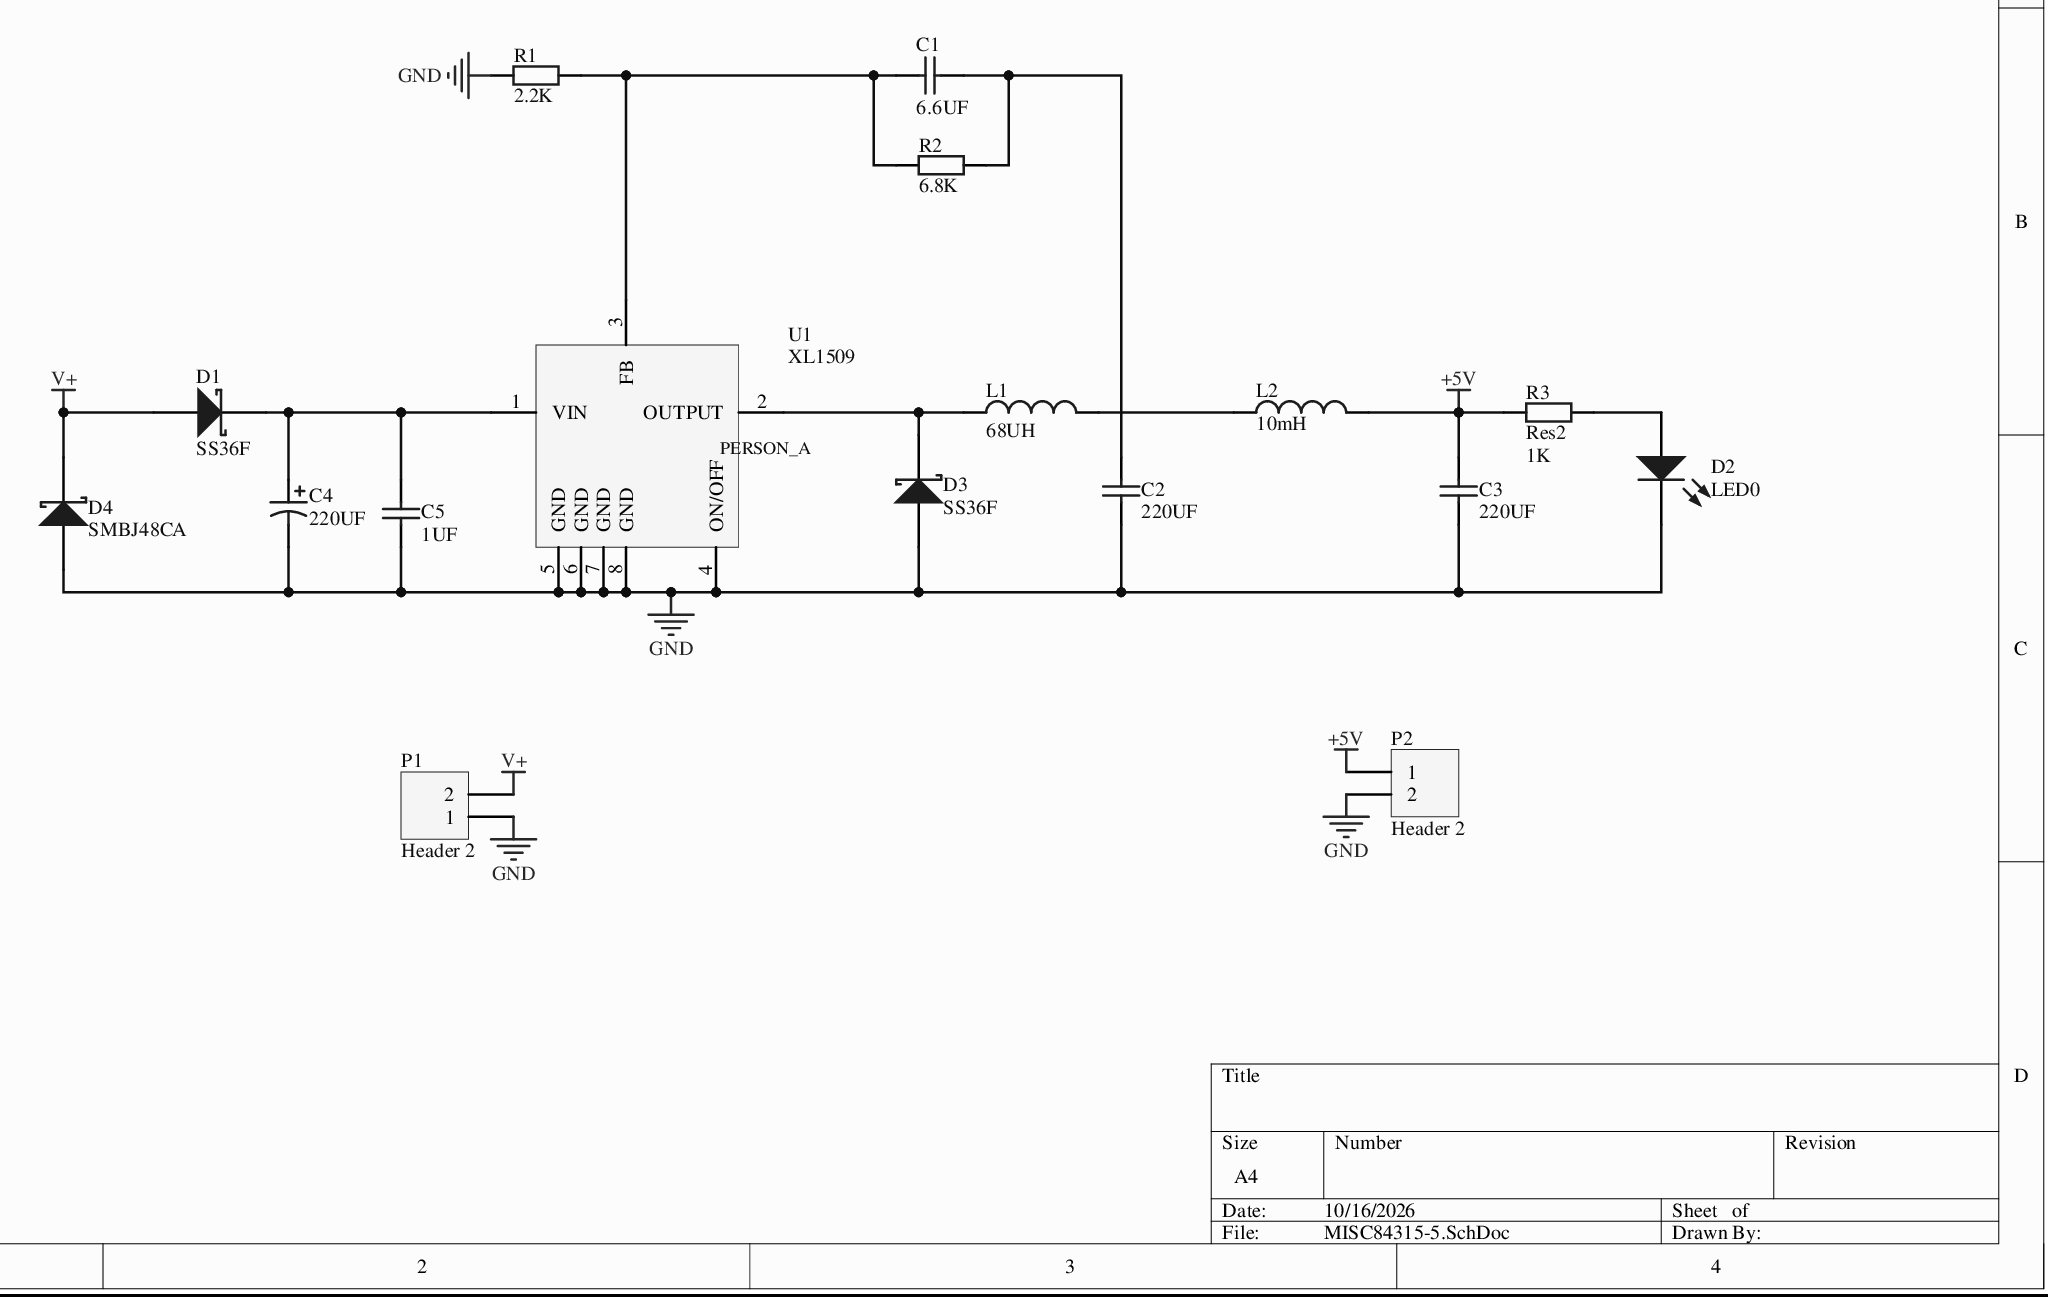
[diagram p0: MISC84315-5.SchDoc]
# Altium project MISC84315-2.PrjPcb
1 sheet, 17 parts. Net scope: global (net labels, ports and power ports of the same name join across sheets).
Board file: MISC84315.PcbDoc

## Sheet MISC84315-5.SchDoc
size A4

### Parts
C1  6.6UF  [C0805]
C2  220UF  [C0805]
C3  220UF  [C0805]
C4  220UF  [RAD-0.4]
C5  1UF  [C0805]
D1  SS36F  [C1206]
D2  LED0  [LED-0]
D3  SS36F  [C1206]
D4  SMBJ48CA  [C1206]
L1  68UH  [INDC1608L]
L2  value 10mH  [INDC1608L]  (hidden comment: Inductor)
P1  Header 2  [HDR1X2]
P2  Header 2  [HDR1X2]
R1  2.2K  [C0805]
R2  6.8K  [C0805]
R3  Res2  value 1K  [C0805]
U1  XL1509  [ESOP8]

### Nets
+5V: C3.2 L2.2 P2.1 R3.1
GND: C2.1 C3.1 C4.2 C5.1 D2.2(K) D3.1(A) D4.1(A) P1.1 P2.2 R1.1 U1.4(ON/OFF) U1.5(GND) U1.6(GND) U1.7(GND) U1.8(GND)
V+: D1.1(A) D4.2(K) P1.2
NetC1_1: C1.1 R1.2 R2.1 U1.3(FB)
NetC1_2: C1.2 C2.2 R2.2
NetC4_1: C4.1 C5.2 D1.2(K) U1.1(VIN)
NetD2_1: D2.1(A) R3.2
NetD3_2: D3.2(K) L1.1 U1.2(OUTPUT)
NetL1_2: L1.2 L2.1

### Library data of the parts
C1-C3 C5 = Cap: Capacitor; Value: 100pF; Published: 8-Jun-2000; LatestRevisionDate: 17-Jul-2002; LatestRevisionNote: Re-released for DXP Platform.; PackageReference: RAD-0.3; PackageDescription: Radial Cap, Thru-Hole; 2 Leads; 0.3 in Pin Spacing; Publisher: Altium Limited
C4 = Cap Pol1: Polarized Capacitor (Radial); Value: 100pF; Published: 8-Jun-2000; LatestRevisionDate: 17-Jul-2002; LatestRevisionNote: Re-released for DXP Platform.; PackageReference: RB7.6-15; PackageDescription: Polarized Capacitor (Radial); 2 Leads; Publisher: Altium Limited
D1 D3 D4 = D Schottky: Schottky Diode; Published: 8-Jun-2000; LatestRevisionDate: 17-Jul-2002; LatestRevisionNote: Re-released for DXP Platform.; PackageReference: SMB; PackageDescription: DO-214-AA/SMB; 2 C-Bend Leads; Body 5.3 x 3.6 mm, inc. leads (LxW); Code_JEDEC: DO-214-AA; Publisher: Altium Limited
D2 = LED0: Typical INFRARED GaAs LED; Published: 8-Jun-2000; LatestRevisionDate: 08-Jul-2005; LatestRevisionNote: Mech Layer 1 removed.; PackageReference: LED-0; PackageDescription: LED; 2 Leads; Publisher: Altium Limited
L1 = Inductor: Code_IEC: 1005; Value: 10mH; Published: 8-Jun-2000; LatestRevisionDate: 29-May-2009; LatestRevisionNote: IPC-7351 Footprint Added.; PackageReference: 0402-A; PackageDescription: Chip Inductor; Code_JEITA: 0402; Publisher: Altium Limited
L2 = Inductor: Code_IEC: 1005; Published: 8-Jun-2000; LatestRevisionDate: 29-May-2009; LatestRevisionNote: IPC-7351 Footprint Added.; PackageReference: 0402-A; PackageDescription: Chip Inductor; Code_JEITA: 0402; Publisher: Altium Limited
P1 P2 = Header 2: Header, 2-Pin; LatestRevisionDate: 17-Jul-2002; LatestRevisionNote: Re-released for DXP Platform.; Publisher: Altium Limited
R1 R2 = Res2: Resistor; Value: 1K; Published: 8-Jun-2000; LatestRevisionDate: 17-Jul-2002; LatestRevisionNote: Re-released for DXP Platform.; PackageReference: AXIAL-0.4; PackageDescription: Axial Device, Thru-Hole; 2 Leads; 0.4 in Pin Spacing; Publisher: Altium Limited
R3 = Res2: Resistor; Published: 8-Jun-2000; LatestRevisionDate: 17-Jul-2002; LatestRevisionNote: Re-released for DXP Platform.; PackageReference: AXIAL-0.4; PackageDescription: Axial Device, Thru-Hole; 2 Leads; 0.4 in Pin Spacing; Publisher: Altium Limited